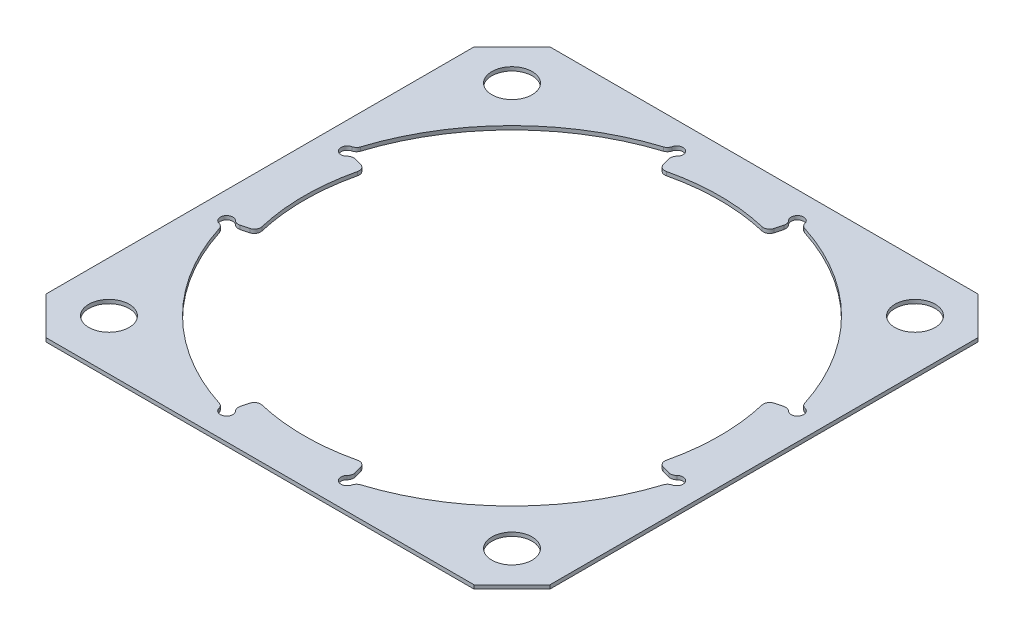
SolidWorks part; units mm, degrees
material "65Mn"
ref_plane "Front Plane" through (0, 0, 0) normal (0, 0, 1) x (1, 0, 0)
ref_plane "Top Plane" through (0, 0, 0) normal (0, 1, 0) x (1, 0, 0)
ref_plane "Right Plane" through (0, 0, 0) normal (1, 0, 0) x (0, 0, -1)
sketch "Sketch1" plane through (0, 0, 0) normal (0, 1, 0) x (1, 0, 0)
  line L0 (-20, 17) -> (-17, 20)
  line L1 (-17, 20) -> (17, 20)
  line L2 (-20, 17) -> (-20, -17)
  line L3 (-17, -20) -> (17, -20)
  line L4 (20, 17) -> (20, -17)
  line L5 (-20, 20) -> (20, -20) construction
  line L6 (-20, -20) -> (20, 20) construction
  line L7 (-20, -17) -> (-17, -20)
  line L8 (17, -20) -> (20, -17)
  line L9 (17, 20) -> (20, 17)
  point P0 (0, 0)
  dimension "D1" = 40
  dimension "D2" = 40
extrude "Boss-Extrude1" add sketch "Sketch1" along normal blind 0.3
sketch "Sketch2" plane through (0, 0.3, 0) normal (0, 1, 0) x (1, 0, 0)
  line L0 (-17.3867, 4.6587) -> (-15.9378, 4.2705)
  line L1 (-15.9378, 4.2705) -> (0, 0) construction
  line L2 (0, 0) -> (-18.5, 0) construction
  line L3 (-17.3867, -4.6587) -> (-15.9378, -4.2705)
  line L4 (4.6587, 17.3867) -> (4.2705, 15.9378)
  line L5 (-4.6587, 17.3867) -> (-4.2705, 15.9378)
  line L6 (17.3867, -4.6587) -> (15.9378, -4.2705)
  line L7 (17.3867, 4.6587) -> (15.9378, 4.2705)
  line L8 (-4.6587, -17.3867) -> (-4.2705, -15.9378)
  line L9 (4.6587, -17.3867) -> (4.2705, -15.9378)
  arc A0 (-17.9925, -4.3035) -> (-4.3035, -17.9925) centre (0, 0) ccw
  arc A1 (-4.2705, -15.9378) -> (4.2705, -15.9378) centre (0, 0) ccw
  arc A2 (-17.9925, 4.3035) -> (-17.3867, 4.6587) centre (-17.8696, 4.7882) ccw
  arc A3 (-17.9925, -4.3035) -> (-17.3867, -4.6587) centre (-17.8696, -4.7882) cw
  arc A4 (4.3035, 17.9925) -> (4.6587, 17.3867) centre (4.7882, 17.8696) ccw
  arc A5 (-4.3035, 17.9925) -> (-4.6587, 17.3867) centre (-4.7882, 17.8696) cw
  arc A6 (17.9925, -4.3035) -> (17.3867, -4.6587) centre (17.8696, -4.7882) ccw
  arc A7 (17.9925, 4.3035) -> (17.3867, 4.6587) centre (17.8696, 4.7882) cw
  arc A8 (-4.3035, -17.9925) -> (-4.6587, -17.3867) centre (-4.7882, -17.8696) ccw
  arc A9 (4.3035, -17.9925) -> (4.6587, -17.3867) centre (4.7882, -17.8696) cw
  arc A10 (4.3035, -17.9925) -> (17.9925, -4.3035) centre (0, 0) ccw
  arc A11 (15.9378, -4.2705) -> (15.9378, 4.2705) centre (0, 0) ccw
  arc A12 (17.9925, 4.3035) -> (4.3035, 17.9925) centre (0, 0) ccw
  arc A13 (4.2705, 15.9378) -> (-4.2705, 15.9378) centre (0, 0) ccw
  arc A14 (-4.3035, 17.9925) -> (-17.9925, 4.3035) centre (0, 0) ccw
  arc A15 (-15.9378, 4.2705) -> (-15.9378, -4.2705) centre (0, 0) ccw
  dimension "D1" = 37
  dimension "D2" = 33
  dimension "D4" = 1
  dimension "D3" = 15
  dimension "D5" = 4
extrude "Cut-Extrude1" cut sketch "Sketch2" against normal blind 0.4
sketch "Sketch3" plane through (0, 0.3, 0) normal (0, 1, 0) x (1, 0, 0)
  line L0 (0, 0) -> (-9.8938, 0) construction
  circle A0 centre (-17.8696, 4.7882) radius 0.5
  circle A1 centre (-17.8696, -4.7882) radius 0.5
  circle A2 centre (4.7882, 17.8696) radius 0.5
  circle A3 centre (-4.7882, 17.8696) radius 0.5
  circle A4 centre (17.8696, -4.7882) radius 0.5
  circle A5 centre (17.8696, 4.7882) radius 0.5
  circle A6 centre (-4.7882, -17.8696) radius 0.5
  circle A7 centre (4.7882, -17.8696) radius 0.5
  dimension "D1" = 1
  dimension "D2" = 4
extrude "Cut-Extrude2" cut sketch "Sketch3" against normal blind 0.4
fillet "Fillet1" radius 0.5 24 edges at (-17.7337, 0.15, 5.2693) (-17.3867, 0.15, 4.6587) (-15.9378, 0.15, 4.2705) (-15.9378, 0.15, -4.2705) (-17.3867, 0.15, -4.6587) (-17.7337, 0.15, -5.2693) (-4.6587, 0.15, -17.3867) (-5.2693, 0.15, -17.7337) (-4.2705, 0.15, -15.9378) (4.2705, 0.15, -15.9378) (4.6587, 0.15, -17.3867) (5.2693, 0.15, -17.7337) (17.3867, 0.15, -4.6587) (17.7337, 0.15, -5.2693) (15.9378, 0.15, -4.2705) (15.9378, 0.15, 4.2705) (17.3867, 0.15, 4.6587) (17.7337, 0.15, 5.2693) (5.2693, 0.15, 17.7337) (4.6587, 0.15, 17.3867) (4.2705, 0.15, 15.9378) (-4.2705, 0.15, 15.9378) (-4.6587, 0.15, 17.3867) (-5.2693, 0.15, 17.7337)
sketch "Sketch4" plane through (0, 0.3, 0) normal (0, 1, 0) x (1, 0, 0)
  line L0 (0, 7.1493) -> (0, 0) construction
  line L1 (0, 0) -> (-7.1778, 0) construction
  circle A0 centre (-16, 16) radius 1.6
  circle A1 centre (16, 16) radius 1.6
  circle A2 centre (16, -16) radius 1.6
  circle A3 centre (-16, -16) radius 1.6
  dimension "D1" = 16
  dimension "D2" = 16
  dimension "D3" = 3.2
extrude "Cut-Extrude3" cut sketch "Sketch4" against normal blind 0.4
